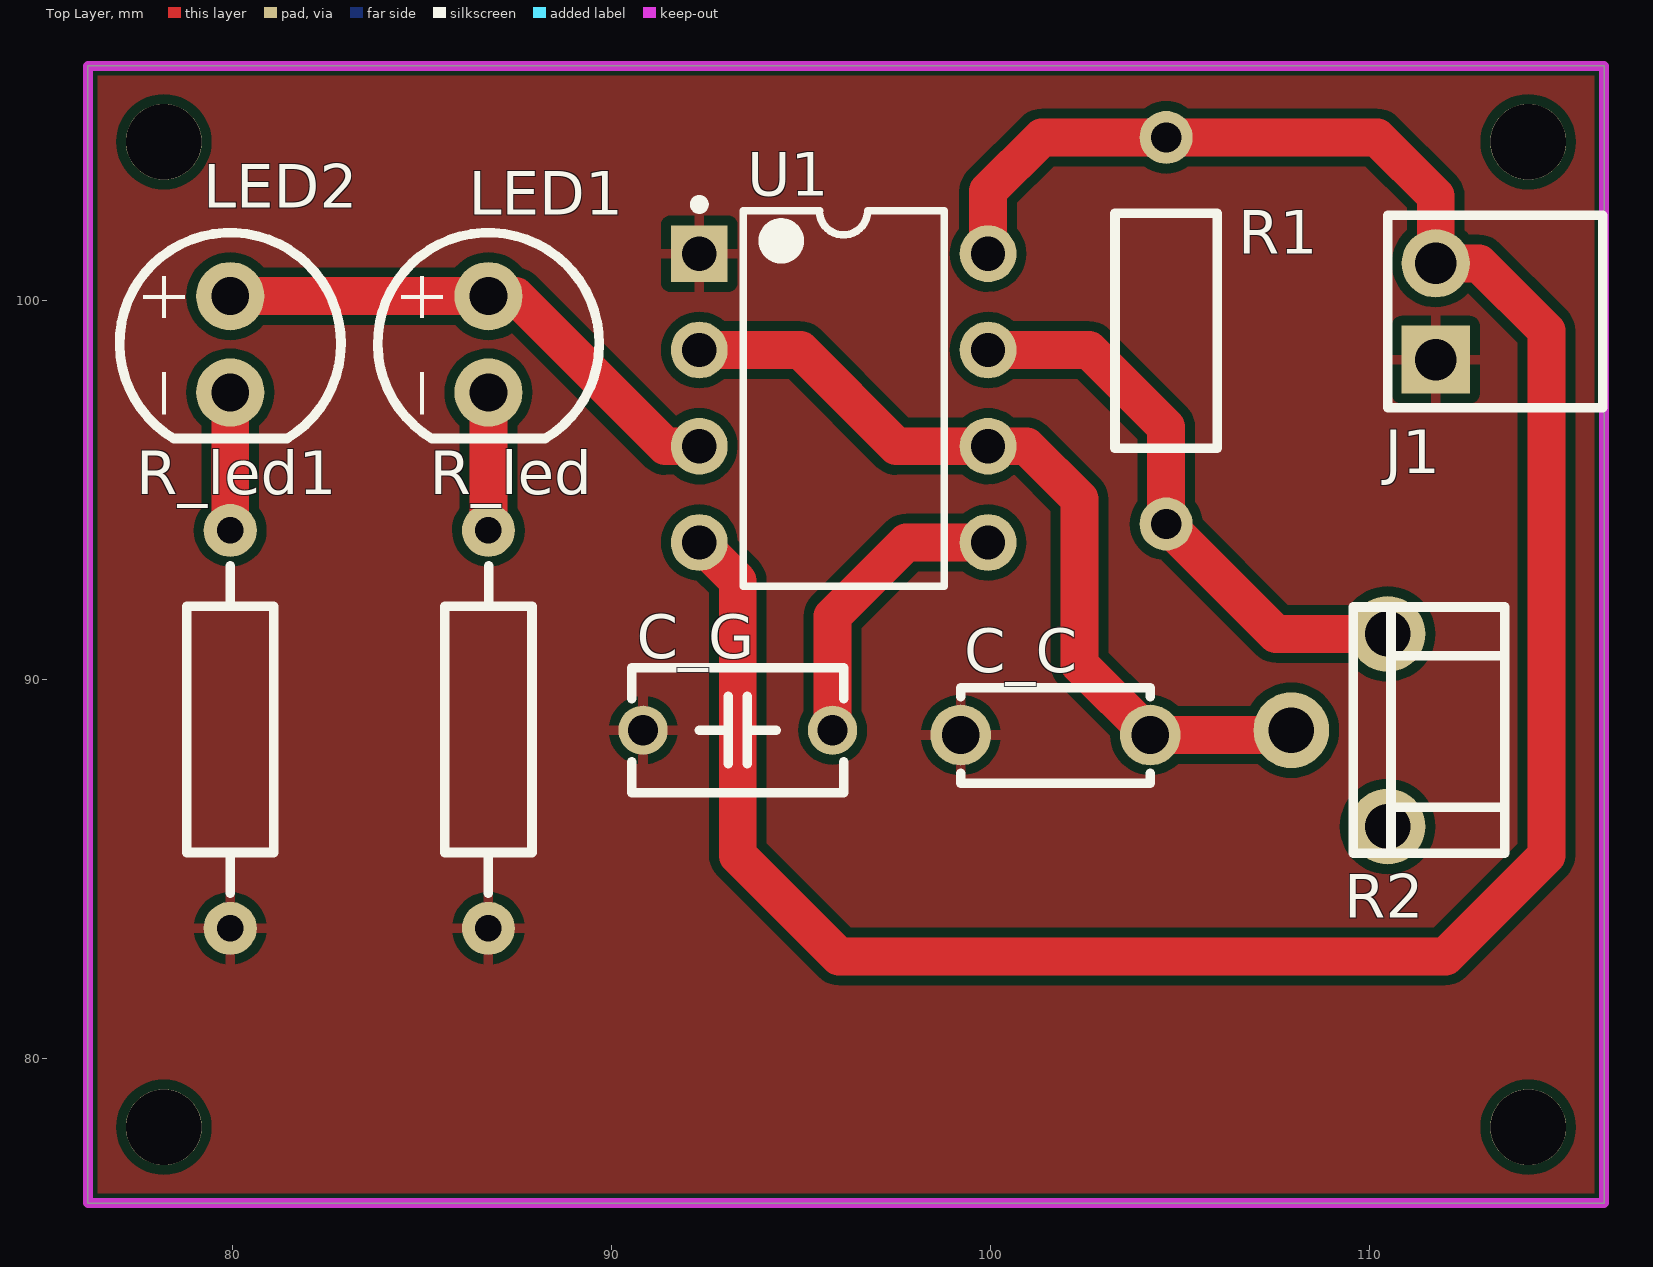
[diagram p0: Top Layer view]
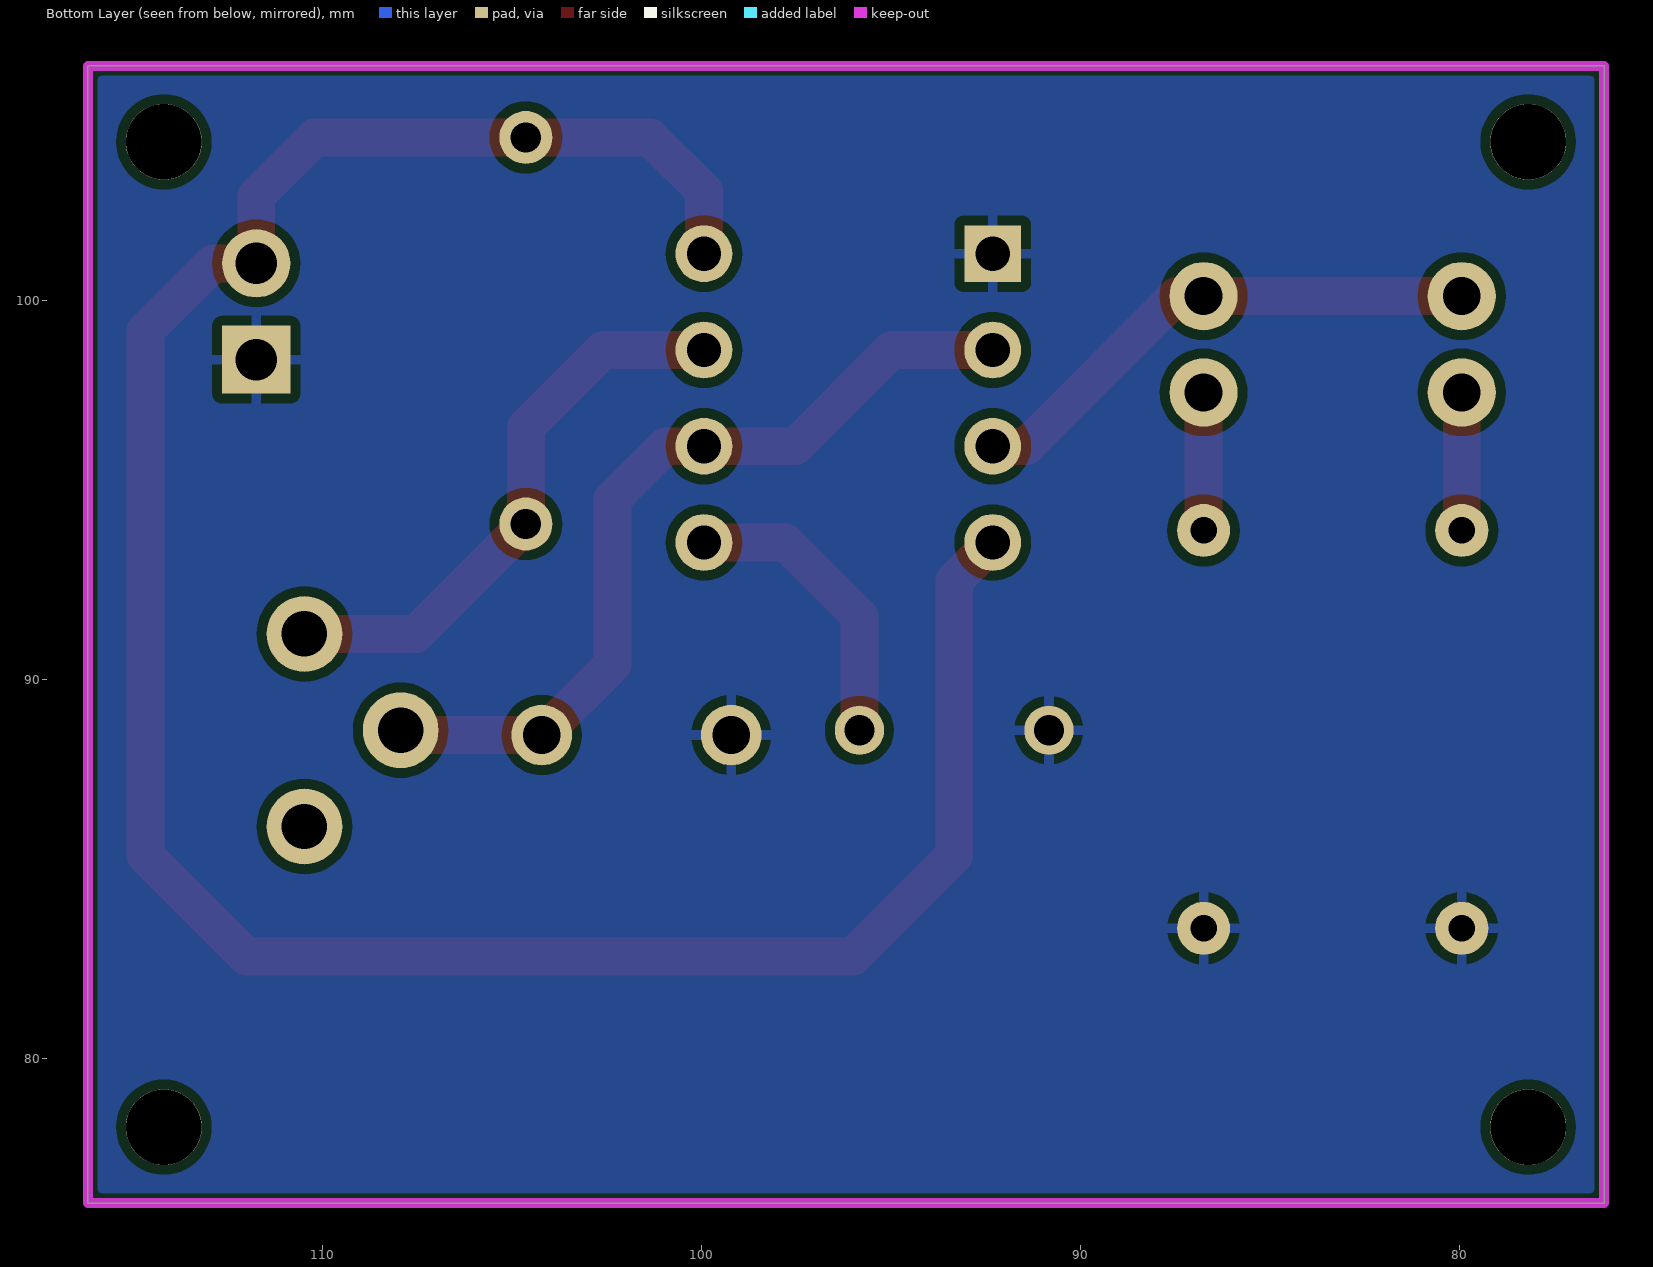
[diagram p1: Bottom Layer view, seen from below]
# Altium PCB MISC49908.pcbdoc
Units mm, origin at the board's own origin, x right, y up, seen from the top; angles counter-clockwise.
Board outline 40 x 30 mm, 2 copper layers (Top Layer, Bottom Layer), stack 1.58 mm thick; 10 components, 8 nets, 31 pads, 0 vias.

## Layer stack, top to bottom
Top Solder Mask Layer: solder mask 0.01, Dk 3.3
Top Layer: signal copper 0.035
Dielectric1: surface 1.51, FR4, Dk 4.5
Bottom Layer: signal copper 0.035
Bottom Solder Mask Layer: solder mask 0.01, Dk 3.3

## Board outline
76.2,106.2 76.2,76.2 116.2,76.2 116.2,106.2

## Design rules (kind name [scope] priority, off if disabled: settings)
BoardOutlineClearance copperThickness2oz_1 [All] p2 off: genericclearance=0.203 ignorepadtopadclearanceinfootprint=FALSE except(0: Arc-SplitContinuation Track-SplitContinuation SMDPad-SplitContinuation THPad-SplitContinuation Via-SplitContinuation Fill-SplitContinuation Region-SplitContinuation Poly-SplitContinuation Text-SplitContinuation Hole-SplitContinuation; 0.152: Arc-CutoutEdge SMDPad-CutoutEdge THPad-CutoutEdge Via-CutoutEdge Fill-CutoutEdge Region-CutoutEdge Text-CutoutEdge; 0.176: Hole-OutlineEdge Hole-CutoutEdge; 0.254: Poly-OutlineEdge Poly-CutoutEdge; 0.3: Arc-OutlineEdge Track-OutlineEdge SMDPad-OutlineEdge THPad-OutlineEdge Via-OutlineEdge Fill-OutlineEdge Region-OutlineEdge Text-OutlineEdge Track-CutoutEdge)
BoardOutlineClearance copperThickness1oz_1 [All] p4: genericclearance=0.102 ignorepadtopadclearanceinfootprint=FALSE except(0: Arc-SplitContinuation Track-SplitContinuation SMDPad-SplitContinuation THPad-SplitContinuation Via-SplitContinuation Fill-SplitContinuation Region-SplitContinuation Poly-SplitContinuation Text-SplitContinuation Hole-SplitContinuation; 0.152: SMDPad-CutoutEdge THPad-CutoutEdge Via-CutoutEdge Fill-CutoutEdge Region-CutoutEdge Text-CutoutEdge; 0.176: Hole-OutlineEdge Hole-CutoutEdge; 0.254: Poly-OutlineEdge Poly-CutoutEdge; 0.3: Arc-OutlineEdge Track-OutlineEdge SMDPad-OutlineEdge THPad-OutlineEdge Via-OutlineEdge Fill-OutlineEdge Region-OutlineEdge Text-OutlineEdge Arc-CutoutEdge Track-CutoutEdge)
Clearance copperThickness2oz [All] p1 off: gap=0.203 ignorepadtopadclearanceinfootprint=FALSE except(0.152: SMDPad-Track SMDPad-SMDPad THPad-Track SMDPad-THPad THPad-THPad Track-Via SMDPad-Via THPad-Via Via-Via Fill-Track Region-Track Fill-SMDPad Region-SMDPad Fill-THPad Region-THPad Fill-Via Region-Via Fill-Fill Fill-Region Region-Region Arc-Track Arc-SMDPad Arc-THPad Arc-Via Fill-Arc Region-Arc Arc-Arc Text-Track SMDPad-Text Text-THPad Text-Via Fill-Text Region-Text Arc-Text Text-Text; 0.176: Hole-Track Hole-SMDPad Hole-THPad Hole-Via Fill-Hole Region-Hole Hole-Arc Hole-Text; 0.254: Poly-Track Poly-SMDPad Poly-THPad Poly-Via Poly-Fill Poly-Region Poly-Poly Poly-Arc Poly-Text Poly-Hole)
Clearance copperThickness1oz [All] p3: gap=0.102 ignorepadtopadclearanceinfootprint=FALSE except(0.152: SMDPad-Track SMDPad-SMDPad THPad-Track SMDPad-THPad THPad-THPad Track-Via SMDPad-Via THPad-Via Via-Via Fill-Track Region-Track Fill-SMDPad Region-SMDPad Fill-THPad Region-THPad Fill-Via Region-Via Fill-Fill Fill-Region Region-Region Arc-Track Arc-SMDPad Arc-THPad Arc-Via Fill-Arc Region-Arc Arc-Arc Text-Track SMDPad-Text Text-THPad Text-Via Fill-Text Region-Text Arc-Text Text-Text; 0.176: Hole-Track Hole-SMDPad Hole-THPad Hole-Via Fill-Hole Region-Hole Hole-Arc Hole-Text; 0.254: Poly-Track Poly-SMDPad Poly-THPad Poly-Via Poly-Fill Poly-Region Poly-Poly Poly-Arc Poly-Text Poly-Hole)
Creepage creepage [All] p1: checkdistance=0 ignoreinternallayers=TRUE applytopolygonpour=TRUE
DiffPairsRouting differentialPair [All] p1: maxlimit=0.152 minlimit=0.152 mostfreqgap=0.152 toplayer_minwidth=0.127 toplayer_prefwidth=0.254 toplayer_maxwidth=2.54 toplayer_mingap=0.152 toplayer_prefgap=0.152 toplayer_maxgap=0.152 bottomlayer_minwidth=0.127 bottomlayer_prefwidth=0.254 bottomlayer_maxwidth=2.54 bottomlayer_mingap=0.152 bottomlayer_prefgap=0.152 bottomlayer_maxgap=0.152 maxuncoupledlength=0.254
HoleToHoleClearance otherClearance [All] p1: gap=0.3 allowstackedmicrovias=TRUE
Length netLength [All] p1: minlimit=0 maxlimit=0
MatchedLengths netLengthTolerance [All] p1: tolerance=25.4
PasteMaskExpansion pasteMaskExpansion [All] p1: expansion=0
PlaneConnect innerPlane [All] p1: planeconnectstyle=Relief reliefexpansion=0.508 reliefentries=4 reliefconductorwidth=0.254 reliefairgap=0.254
PolygonConnect copperRegion [(InNet('GND'))] p1: connectstyle=Relief reliefconductorwidth=0.254 reliefentries=4 polygonreliefangle="90 Angle" airgapwidth=0.254 via.connectstyle=Relief via.reliefconductorwidth=0.254 via.reliefentries=4 via.polygonreliefangle="90 Angle" via.airgapwidth=0.254
RoutingVias viaSize [All] p1: holewidth=0.305 width=0.61 viastyle="Through Hole" minholewidth=0.3 minwidth=0.5 maxholewidth=6.3 maxwidth=10
SolderMaskExpansion solderMaskExpansion [IsVia] p1: expansion=-25.4 istentingtop=TRUE
SolderMaskExpansion solderMaskExpansion [All] p2: expansion=0.051 istentingtop=FALSE
Width copperThickness2oz_2 [All] p1 off: maxlimit=2.54 minlimit=0.203 preferedwidth=0.254
Width copperThickness1oz_2 [All] p2: maxlimit=2.54 minlimit=0.127 preferedwidth=0.254

## Components (designator, comment, footprint, x,y, rotation, side; value= is the part's Value field where it differs from the comment)
C_C "100nF" CAP-TH_L5.0-W2.5-P5.00-D1.0 101.727,88.547 r0 top
C_G "10nF" CAP-TH_L5.5-W3.0-P5.00-D0.6 93.345,88.674 r0 top
J1 "" HDR-TH_2P-P2.54-V-M-1 111.76,99.723 r90 top
LED1 "XL-502SURD" LED-TH_BD5.9-P2.54-RD_RED 86.765,98.857 r90 top
LED2 "XL-502SURD" LED-TH_BD5.9-P2.54-RD_RED 79.953,98.857 r90 top
R1 "1kΩ" RES-TH_BD2.7-L6.2-P10.20-D0.4 104.648,99.215 r90 top
R2 "1MΩ" RES-ADJ-TH_RM063-103 109.22,88.674 r90 top
R_led "470Ω" RES-TH_BD2.3-L6.5-P10.50-D0.5 86.765,88.697 r90 top
R_led1 "470Ω" RES-TH_BD2.3-L6.5-P10.50-D0.5 79.953,88.697 r90 top
U1 "NE555P" DIP-8_L9.8-W6.6-P2.54-LS7.6-BL 96.139,97.437 r270 top

## Footprints (in the part's own frame and the unit in brackets; to place one, negate y for a bottom-side part, rotate by r counter-clockwise, add the part's x,y. Pads: shape width x height; smd on the part's side, far side on the other; paste and mask are expansions set on the pad)
CAP-TH_L5.0-W2.5-P5.00-D1.0 [mm]
  round 1.6 hole 1: 1(-2.5,0) 2(2.5,0)
  silkscreen extent -2.5,-1.27 2.5,1.25
CAP-TH_L5.5-W3.0-P5.00-D0.6 [mm]
  round 1.3 hole 0.8 paste+0 mask+0.05: 1(-2.5,0) 2(2.5,0)
  silkscreen extent -2.79,-1.65 2.79,1.65
DIP-8_L9.8-W6.6-P2.54-LS7.6-BL [mm]
  rect 1.5x1.5 hole 0.9: 1(-3.81,-3.81)
  round 1.5 hole 0.9: 2(-1.27,-3.81) 3(1.27,-3.81) 4(3.81,-3.81) 5(3.81,3.81) 6(1.27,3.81) 7(-1.27,3.81) 8(-3.81,3.81)
  silkscreen extent -5.23,-3.93 4.96,2.65
HDR-TH_2P-P2.54-V-M-1 [mm]
  rect 1.8x1.8 hole 1.1: 1(-1.27,0)
  round 1.8 hole 1.1: 2(1.27,0)
  silkscreen extent -2.54,-4.41 2.54,1.27
LED-TH_BD5.9-P2.54-RD_RED [mm]
  round 1.8 hole 1 paste+0 mask+0.05: 1(-1.27,0) 2(1.27,0)
  silkscreen extent -2.49,-2.92 2.94,2.92
RES-ADJ-TH_RM063-103 [mm]
  round 2 hole 1.2 paste+0 mask+0.05: 1(-2.54,-1.27) 2(0,1.27) 3(2.54,-1.27)
  silkscreen extent -3.25,-4.36 3.25,-0.36
RES-TH_BD2.3-L6.5-P10.50-D0.5 [mm]
  round 1.4 hole 0.7: 1(-5.25,0) 2(5.25,0)
  silkscreen extent -4.32,-1.15 4.32,1.15
RES-TH_BD2.7-L6.2-P10.20-D0.4 [mm]
  round 1.4 hole 0.8 copper offset 0,0: 1(-5.1,0) 2(5.1,0)
  silkscreen extent -3.1,-1.35 3.1,1.35

## Free pads (board coordinates)
  round 2 hole 2: 1(78.2,78.2) 1(78.2,104.2) 1(114.2,78.2) 1(114.2,104.2)

## Nets (pads, with @x,y where several pads share a name; then routed paths per layer and width w, separated by ;. In a path a pad name is that pad's centre, name@x,y a point inside that pad or via, vN(x,y) a via of type N, cw(c..) or ccw(c..) an arc to the next point about the centre after c; other vN are vias at no path point)
$1N34: C_G.2 U1.5 | length 7.9
  Top Layer w1: C_G.2 95.845,91.682 97.79,93.627 U1.5
$1N35: C_C.2 R2.2 U1.2 U1.6 | length 22.4
  Top Layer w1: U1.2 94.996,98.707 97.536,96.167 U1.6 100.965,96.167 102.362,94.77 102.362,90.412 C_C.2 107.823,88.547 R2.2
$1N36: R1.1 R2.3 U1.7 | length 15.1
  Top Layer w1: U1.7 102.616,98.707 104.648,96.675 R1.1 107.549,91.214 R2.3
$1N39: LED1.2 LED2.2 U1.3 | length 14
  Top Layer w1: LED2.2 LED1.2 87.48,100.127 91.44,96.167 U1.3
$1N41: LED1.1 R_led.2 | length 3.6
  Top Layer w1: R_led.2 LED1.1
$1N43: LED2.1 R_led1.2 | length 3.6
  Top Layer w1: R_led1.2 LED2.1
+5V: J1.2 R1.2 U1.4 U1.8 | length 66.2
  Top Layer w1: U1.4 93.345,92.611 93.345,85.372 96.012,82.705 112.014,82.705 114.681,85.372 114.681,99.215 112.903,100.993 J1.2 111.76,102.771 110.216,104.315 R1.2 101.366,104.315 99.949,102.898 U1.8
GND: C_C.1 C_G.1 J1.1 R_led1.1 R_led.1 U1.1
pads on no net: R2.1

## Polygon pours and split planes (outlines as drawn)
GND on Top Layer (solid, remove dead copper, pour order 0): 76.2,106.2 76.2,76.2 116.2,76.2 116.2,106.2
GND on Bottom Layer (solid, remove dead copper, pour order 2): 76.2,106.2 76.2,76.2 116.2,76.2 116.2,106.2

## Keep-outs
Board Outline Layer:
  the board outline again, w0.254